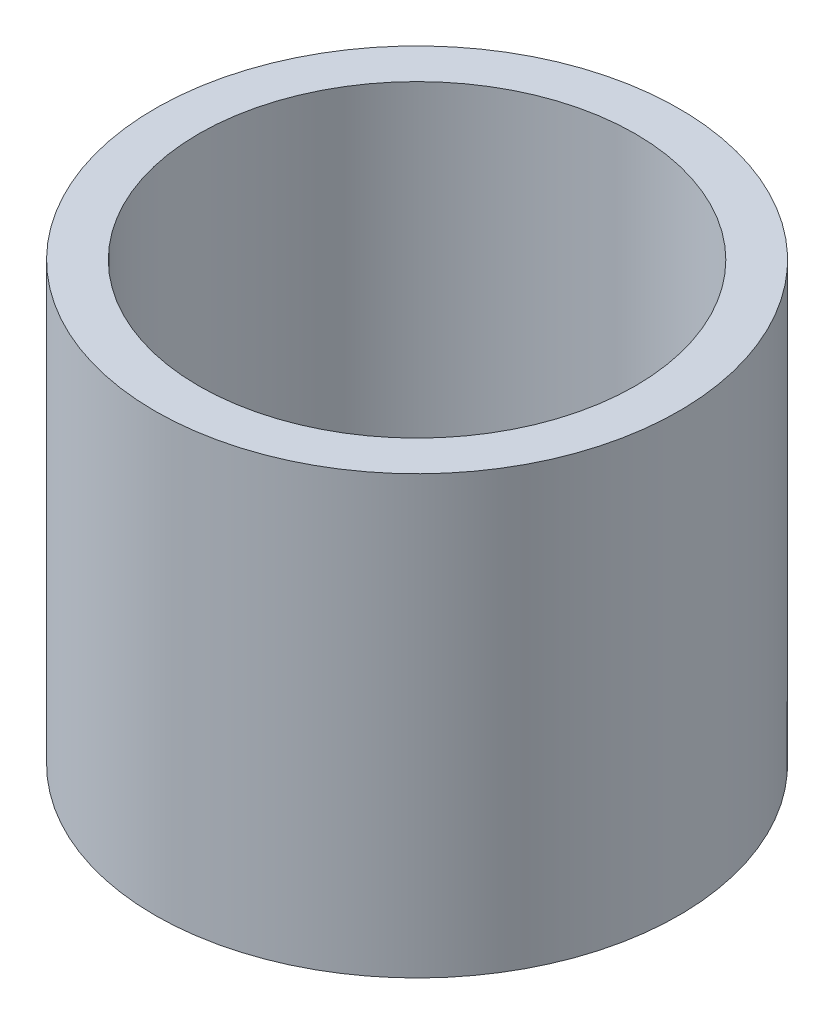
SolidWorks part; units mm, degrees
ref_plane "Front Plane" through (0, 0, 0) normal (0, 0, 1) x (1, 0, 0)
ref_plane "Top Plane" through (0, 0, 0) normal (0, 1, 0) x (1, 0, 0)
ref_plane "Right Plane" through (0, 0, 0) normal (1, 0, 0) x (0, 0, -1)
other "Configuration Table"
sketch "Sketch1" plane through (0, 0, 0) normal (0, 1, 0) x (1, 0, 0)
  circle A0 centre (0, 0) radius 2.5
  circle A1 centre (0, 0) radius 3
  dimension "D1" = 5
  dimension "D2" = 6
extrude "Boss-Extrude1" add sketch "Sketch1" along normal blind 5
